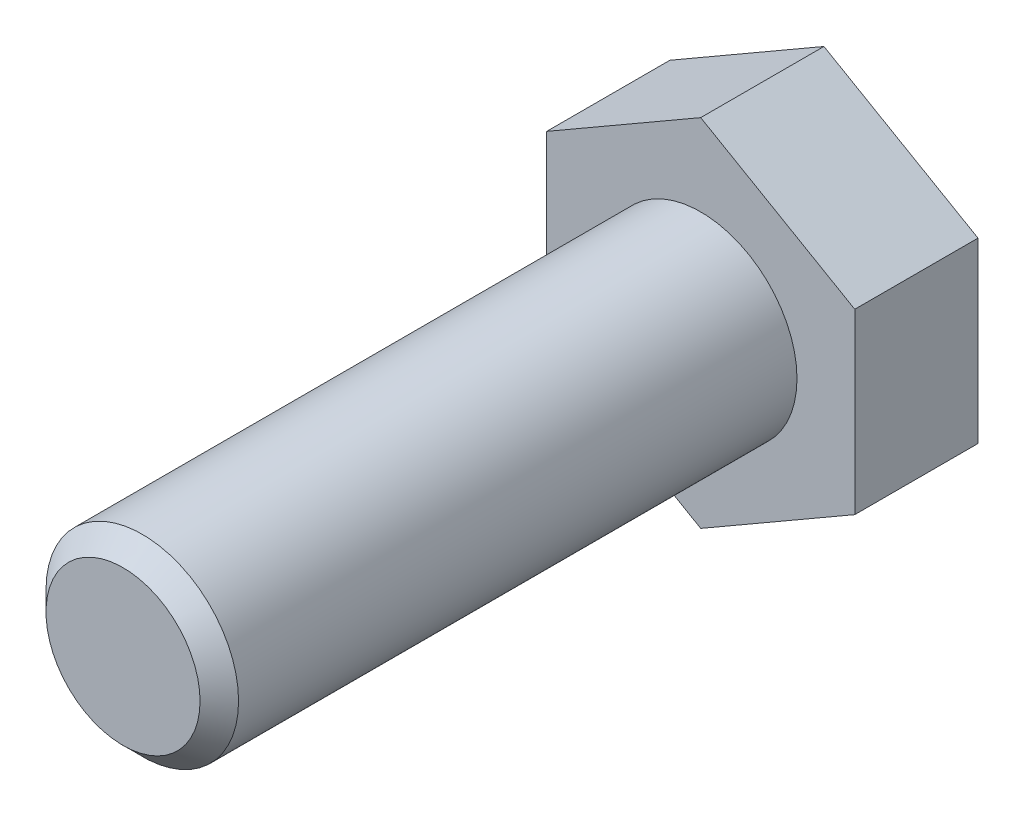
from build123d import *

# Parameters (mm, degrees)
BOSS_EXTRUDE1_DEPTH = 6.4
SKETCH3_R           = 5
BOSS_EXTRUDE2_DEPTH = 30
CHAMFER1_SIZE       = 1


with BuildPart() as part:
    # Sketch1 → Boss-Extrude1 (new body)
    with BuildSketch(Plane.XY):
        Polygon((8, 4.618802154), (0, 9.237604307), (-8, 4.618802154), (-8, -4.618802154), (0, -9.237604307), (8, -4.618802154), align=None)
    extrude(amount=BOSS_EXTRUDE1_DEPTH)

    # Sketch3 → Boss-Extrude2 (add)
    with BuildSketch(Plane.XY.offset(6.4)):
        Circle(SKETCH3_R)
    extrude(amount=BOSS_EXTRUDE2_DEPTH)

    # Chamfer1
    chamfer1_edges = [part.edges().sort_by_distance(p)[0] for p in [
        (-5, 0, 36.4),
    ]]
    chamfer(chamfer1_edges, length=CHAMFER1_SIZE)


solid = part.part
